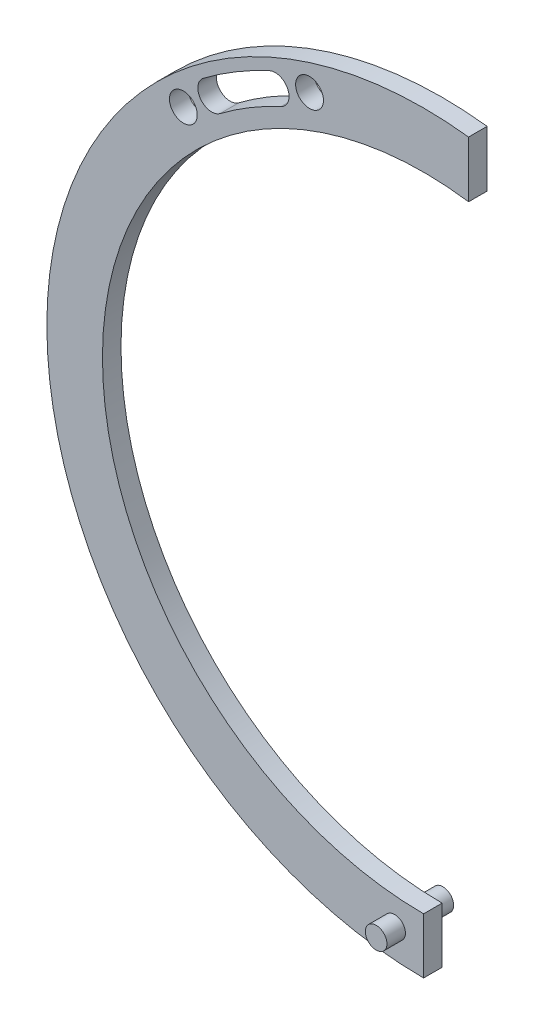
from build123d import *

# Parameters (mm, degrees)
BOSS_EXTRUDE1_DEPTH      = 10
BOSS_EXTRUDE2_DEPTH      = 10
BOSS_EXTRUDE2_DEPTH_BACK = 26
SKETCH2_R                = 5.820264096
CUT_EXTRUDE1_DEPTH       = 629.17046577
CUT_EXTRUDE1_DEPTH_BACK  = 629.17046577
SKETCH3_R                = 7.5


with BuildPart() as part:
    # Sketch1 → Boss-Extrude1 (new body)
    with BuildSketch(Plane.XY):
        with BuildLine():
            Line((-267.317020812, 384.57192575), (-267.301609192, 354.315771574))
            ThreePointArc((-267.301609192, 354.315771574), (-464.45214838, 194.902560898), (-291.585214163, 9.435771703))
            Line((-291.585214163, 9.435771703), (-291.585214163, -20.564228297))
            ThreePointArc((-291.585214163, -20.564228297), (-494.516390011, 194.886544), (-267.317020812, 384.57192575))
        make_face()
    extrude(amount=-BOSS_EXTRUDE1_DEPTH)

    # Sketch2 → Boss-Extrude2 (add, two sides: drawn at the far end of the back side and taken through both)
    with BuildSketch(Plane.XY.offset(-BOSS_EXTRUDE2_DEPTH_BACK)):
        with Locations((-307.201523558, -4.519874966)):
            Circle(SKETCH2_R)
    extrude(amount=BOSS_EXTRUDE2_DEPTH + BOSS_EXTRUDE2_DEPTH_BACK)

    # Sketch3 → Cut-Extrude1 (cut, two sides: drawn at the far end of the back side and taken through both)
    with BuildSketch(Plane.XY.offset(-CUT_EXTRUDE1_DEPTH_BACK)):
        with Locations(Location((-421.223956701, 321.632808197, 0), (0, 0, 180))):
            Circle(SKETCH3_R)
        with Locations(Location((-353.128945359, 362.487113382, 0), (0, 0, 180))):
            Circle(SKETCH3_R)
        with BuildLine():
            ThreePointArc((-374.845259184, 361.822893879), (-393.201425865, 352.083570004), (-410.432690408, 340.469492039))
            ThreePointArc((-410.432690408, 340.469492039), (-411.909575924, 329.966215923), (-401.406299807, 328.489330407))
            ThreePointArc((-401.406299807, 328.489330407), (-385.4837389, 339.221326502), (-368.521711461, 348.220954892))
            ThreePointArc((-368.521711461, 348.220954892), (-364.882515829, 358.183698247), (-374.845259184, 361.822893879))
        make_face()
    extrude(amount=CUT_EXTRUDE1_DEPTH + CUT_EXTRUDE1_DEPTH_BACK, mode=Mode.SUBTRACT)


solid = part.part
